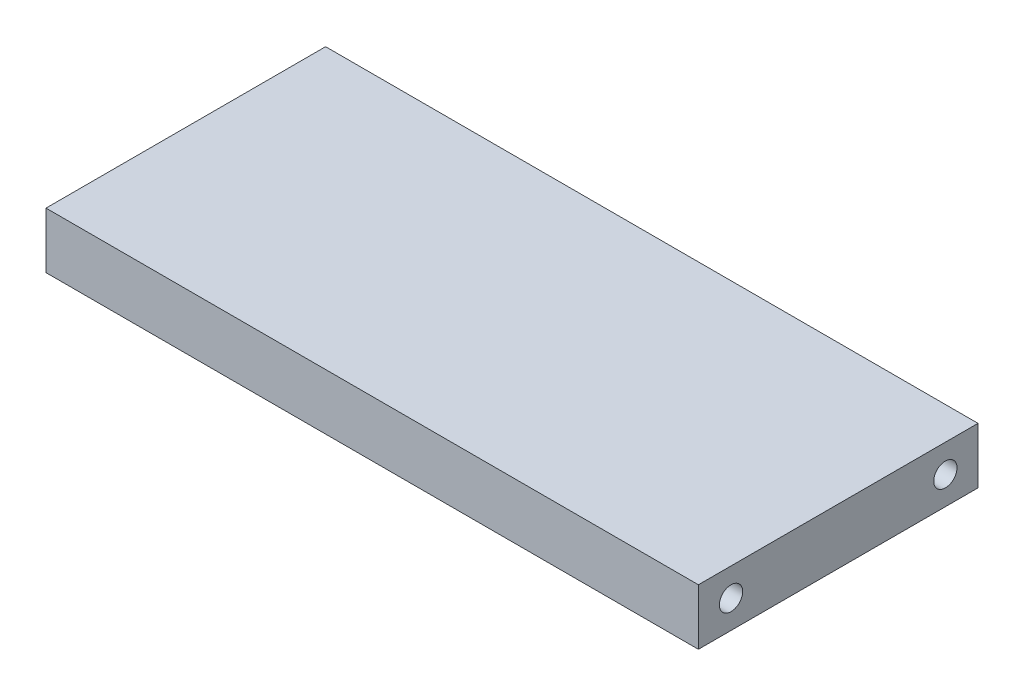
from build123d import *

# Parameters (mm, degrees)
SKETCH1_W           = 70
SKETCH1_H           = 30
BOSS_EXTRUDE1_DEPTH = 6
SKETCH2_R           = 1.25
CUT_EXTRUDE1_DEPTH  = 5
CUT_EXTRUDE2_START  = -5
SKETCH3_R           = 1.25
CUT_EXTRUDE2_DEPTH  = 5


with BuildPart() as part:
    # Sketch1 → Boss-Extrude1 (new body)
    with BuildSketch(Plane(origin=(0, 0, 0), x_dir=(1, 0, 0), z_dir=(0, 1, 0))):
        Rectangle(SKETCH1_W, SKETCH1_H)
    extrude(amount=BOSS_EXTRUDE1_DEPTH)

    # Sketch2 → Cut-Extrude1 (cut)
    with BuildSketch(Plane(origin=(35, 0, 0), x_dir=(0, 0, -1), z_dir=(1, 0, 0))):
        with Locations((11.5, 3)):
            Circle(SKETCH2_R)
        with Locations((-11.5, 3)):
            Circle(SKETCH2_R)
    extrude(amount=-CUT_EXTRUDE1_DEPTH, mode=Mode.SUBTRACT)

    # Sketch3 → Cut-Extrude2 (cut)
    with BuildSketch(Plane.ZY.offset(35).offset(CUT_EXTRUDE2_START)):
        with Locations(Location((-11.5, 3, 0), (0, 0, 180))):
            Circle(SKETCH3_R)
        with Locations(Location((11.5, 3, 0), (0, 0, 180))):
            Circle(SKETCH3_R)
    extrude(amount=CUT_EXTRUDE2_DEPTH, mode=Mode.SUBTRACT)


solid = part.part
